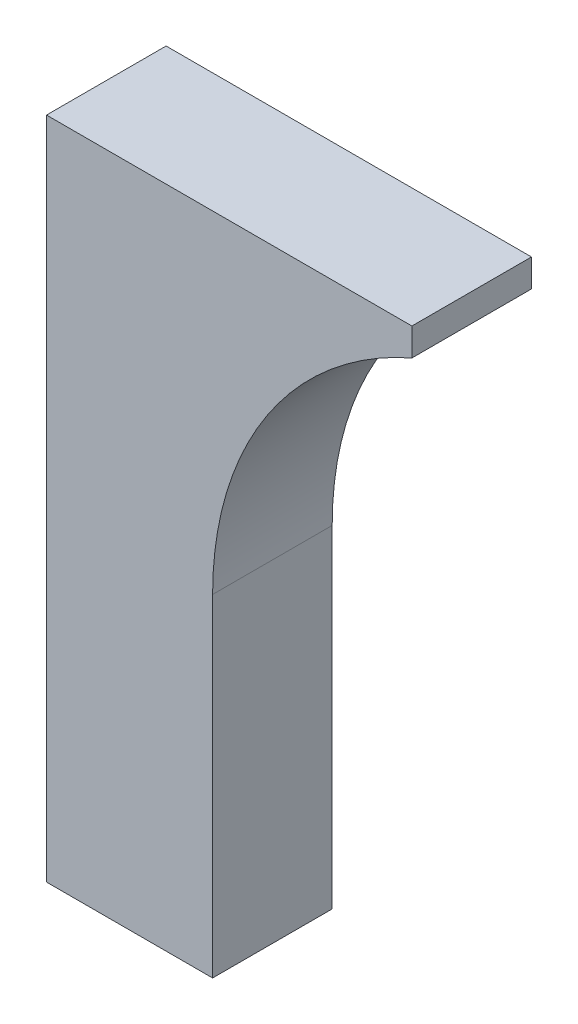
from build123d import *

# Parameters (mm, degrees)
BOSS_EXTRUDE1_DEPTH = 18


with BuildPart() as part:
    # Sketch1 → Boss-Extrude1 (new body)
    with BuildSketch(Plane.XY):
        with BuildLine():
            Line((0, 0), (0, 100))
            Line((0, 100), (55, 100))
            Line((55, 100), (55, 95.82575695))
            ThreePointArc((55, 95.82575695), (33.166998673, 77.386127875), (25, 50))
            Line((25, 50), (25, 0))
            Line((25, 0), (0, 0))
        make_face()
    extrude(amount=BOSS_EXTRUDE1_DEPTH)


solid = part.part
